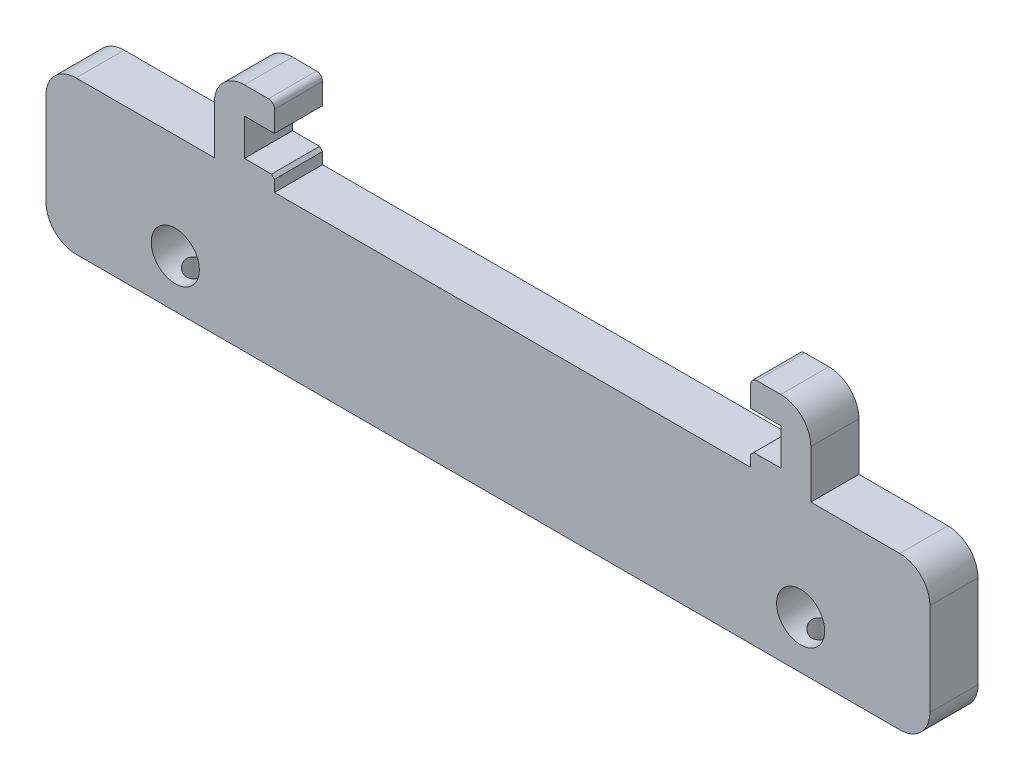
SolidWorks part; units mm, degrees
ref_plane "Front Plane" through (0, 0, 0) normal (0, 0, 1) x (1, 0, 0)
ref_plane "Top Plane" through (0, 0, 0) normal (0, 1, 0) x (1, 0, 0)
ref_plane "Right Plane" through (0, 0, 0) normal (1, 0, 0) x (0, 0, -1)
other "Configuration Table"
sketch "Sketch1" plane through (0, 0, 0) normal (0, 0, 1) x (1, 0, 0)
  line L1 (0, 0) -> (147, 0)
  line L2 (0, 0) -> (0, -25.4)
  line L3 (0, -25.4) -> (147, -25.4)
  line L4 (147, 0) -> (147, -25.4)
  dimension "D1" = 147
  dimension "D2" = 25.4
extrude "Boss-Extrude1" add sketch "Sketch1" along normal blind 8
sketch "Sketch2" plane through (0, 0, 0) normal (0, 1, 0) x (1, 0, 0)
  line L0 (147, 0) -> (0, 0) construction
  line L1 (122.2, 0) -> (127.2, 0)
  line L2 (122.2, 0) -> (122.2, -8)
  line L3 (122.2, -8) -> (127.2, -8)
  line L4 (127.2, 0) -> (127.2, -8)
  line L5 (147, -8) -> (0, -8) construction
  line L7 (0, -8) -> (0, 0) construction
  line L8 (28, 0) -> (33, 0)
  line L9 (28, 0) -> (28, -8)
  line L10 (28, -8) -> (33, -8)
  line L11 (33, 0) -> (33, -8)
  dimension "D1" = 28
  dimension "D2" = 5
  dimension "D3" = 89.2
  dimension "D4" = 5
extrude "Boss-Extrude2" add sketch "Sketch2" along normal blind 10
sketch "Sketch3" plane through (33, 0, 0) normal (1, 0, 0) x (0, 0, -1)
  line L0 (0, 10) -> (0, 0) construction
  line L1 (-8, 10) -> (0, 10)
  line L2 (-8, 10) -> (-8, 8.5)
  line L3 (-8, 8.5) -> (0, 8.5)
  line L4 (0, 10) -> (0, 8.5)
  dimension "D1" = 1.5
extrude "Boss-Extrude3" add sketch "Sketch3" along normal blind 5
ref_plane "Plane1" through (77.6, 0, 0) normal (1, 0, 0) x (0, 0, -1)
mirror "Mirror1" about plane through (77.6, 0, 0) normal (1, 0, 0) of "Boss-Extrude3"
sketch "Sketch4" plane through (0, 0, 0) normal (0, 1, 0) x (1, 0, 0)
  line L0 (38, 0) -> (28, 0) construction
  line L1 (33, 0) -> (38, 0)
  line L2 (33, 0) -> (33, -8)
  line L3 (33, -8) -> (38, -8)
  line L4 (38, 0) -> (38, -8)
  line L5 (122.2, -8) -> (33, -8) construction
  line L6 (38, 0) -> (38, -8) construction
  line L8 (117.2, 0) -> (122.2, 0)
  line L9 (117.2, 0) -> (117.2, -8)
  line L10 (117.2, -8) -> (122.2, -8)
  line L11 (122.2, 0) -> (122.2, -8)
extrude "Boss-Extrude4" add sketch "Sketch4" along normal blind 2.4
sketch "Sketch7" plane through (0, 0, 8) normal (0, 0, 1) x (1, 0, 0)
  line L0 (0, 0) -> (0, -25.4) construction
  line L2 (147, -25.4) -> (147, 0) construction
  line L3 (0, -25.4) -> (147, -25.4) construction
  circle A0 centre (21.5, -17.4) radius 4
  circle A1 centre (125.5, -17.4) radius 4
  dimension "D1" = 8
  dimension "D2" = 8
  dimension "D3" = 104
  dimension "D4" = 21.5
  dimension "D5" = 8
extrude "Cut-Extrude1" cut sketch "Sketch7" against normal through all
sketch "Sketch8" plane through (0, 10, 0) normal (0, 1, 0) x (1, 0, 0)
  line L4 (28, 0) -> (28, -8)
  line L5 (28, -8) -> (38, -8)
  line L6 (38, -8) -> (38, 0)
  line L7 (38, 0) -> (28, 0)
  line L8 (28, 0) -> (28, -8)
  line L9 (28, -8) -> (38, -8)
  line L10 (38, -8) -> (38, 0)
  line L11 (38, 0) -> (28, 0)
  line L12 (127.2, 0) -> (117.2, 0)
  line L13 (117.2, 0) -> (117.2, -8)
  line L14 (117.2, -8) -> (127.2, -8)
  line L15 (127.2, -8) -> (127.2, 0)
  line L16 (127.2, 0) -> (117.2, 0)
  line L17 (117.2, 0) -> (117.2, -8)
  line L18 (117.2, -8) -> (127.2, -8)
  line L19 (127.2, -8) -> (127.2, 0)
  dimension "D1" = 0
  dimension "D2" = 0
extrude "Boss-Extrude5" add sketch "Sketch8" along normal blind 3
fillet "Fillet1" radius 5 4 edges at (0, 0, 4) (147, 0, 4) (127.2, 13, 4) (28, 13, 4)
chamfer "Chamfer1" distance 0.5 angle 45 2 edges at (117.2, 2.4, 4) (38, 2.4, 4)
sketch "Sketch10" plane through (0, -25.4, 0) normal (0, -1, 0) x (1, 0, 0)
  line L0 (0, 8) -> (0, 0) construction
  line L2 (147, 8) -> (147, 0) construction
  point P0 (21.5, 4)
  point P1 (125.5, 4)
  point P4 (0, 4)
  point P7 (147, 4)
  dimension "D1" = 21.5
  dimension "D2" = 21.5
hole_wizard "Ø4.2 (4.2) Diameter Hole1" positions "Sketch10" profile "Sketch11" hole size "Ø4.2" standard "GB"
sketch "Sketch11" plane through (21.5, -25.4, 4) normal (1, 0, 0) x (0, 0, -1)
  line L0 (0, 0) -> (0, 10.7618)
  line L1 (0, 10.7618) -> (2.1, 9.5)
  line L2 (2.1, 9.5) -> (2.1, 0)
  line L5 (2.1, 0) -> (0, 0)
  line L10 (0, 10.7618) -> (-2.1, 9.5) construction
  line L11 (0, -6.35) -> (0, 107.95) construction
  dimension "孔直径" = 4.2
  dimension "孔深度" = 9.5
  dimension "导头角度" = 118
fillet "Fillet2" radius 5 2 edges at (147, -25.4, 4) (0, -25.4, 4)
fillet "Fillet3" radius 1 2 edges at (117.2, 13, 4) (38, 13, 4)
